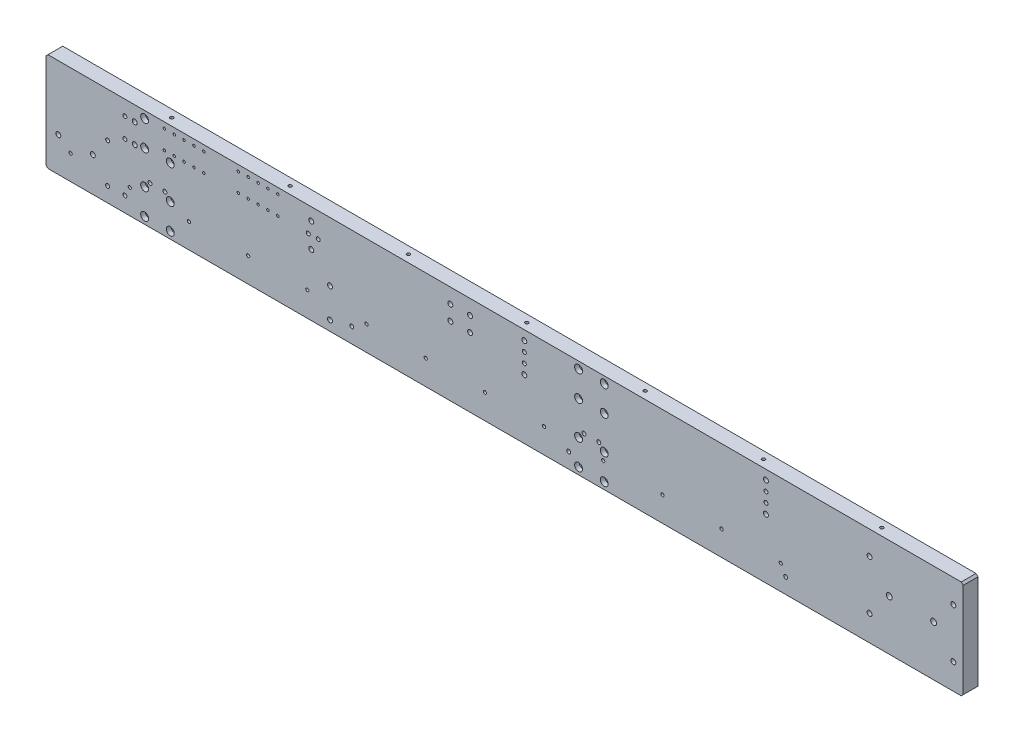
from build123d import *

# Parameters (mm, degrees)
SKETCH2_W                                        = 930
SKETCH2_H                                        = 100
BOSS_EXTRUDE1_DEPTH                              = 15
HOLE_SIZE_PER_HEX_SOCKET_SCREW_TYPE1_D           = 4.5
HOLE_SIZE_PER_HEX_SOCKET_SCREW_TYPE1_CBORE_D     = 8
HOLE_SIZE_PER_HEX_SOCKET_SCREW_TYPE1_CBORE_DEPTH = 4.6
M6_TAPPED_HOLE1_D                                = 5
M6_TAPPED_HOLE1_DEPTH                            = 15
M6_TAPPED_HOLE1_TIP                              = 1.502151548
M6_TAPPED_HOLE2_D                                = 5
M6_TAPPED_HOLE2_DEPTH                            = 15
M6_TAPPED_HOLE2_TIP                              = 1.502151548
LPATTERN2_COUNT                                  = 13
LPATTERN2_PITCH                                  = 60
M3_TAPPED_HOLE1_D                                = 2.5
M3_TAPPED_HOLE1_DEPTH                            = 8.5
M3_TAPPED_HOLE1_TIP                              = 0.751075774
F_4_0_4_DIAMETER_HOLE1_D                         = 4
F_4_0_4_DIAMETER_HOLE1_DEPTH                     = 15
F_4_0_4_DIAMETER_HOLE1_TIP                       = 1.201721238
F_6_0_6_DIAMETER_HOLE1_D                         = 6
F_6_0_6_DIAMETER_HOLE1_DEPTH                     = 15
F_6_0_6_DIAMETER_HOLE1_TIP                       = 1.802581857
M4_TAPPED_HOLE2_D                                = 3.3
M4_TAPPED_HOLE2_DEPTH                            = 11.5
M4_TAPPED_HOLE2_TIP                              = 0.991420021
M4_TAPPED_HOLE3_D                                = 3.3
M4_TAPPED_HOLE3_DEPTH                            = 10.1
M4_TAPPED_HOLE3_TIP                              = 0.991420021
M3_TAPPED_HOLE2_D                                = 2.5
M3_TAPPED_HOLE2_DEPTH                            = 8.5
M3_TAPPED_HOLE2_TIP                              = 0.751075774
CHAMFER1_SIZE                                    = 2


with BuildPart() as part:
    # Sketch2 → Boss-Extrude1 (new body)
    with BuildSketch(Plane.XY):
        with Locations((465, 50)):
            Rectangle(SKETCH2_W, SKETCH2_H)
    extrude(amount=-BOSS_EXTRUDE1_DEPTH)

    # Hole size per hex socket screw type1 (through all)
    with Locations(Plane.XY):
        with Locations((100, 33), (126, 33), (100, 7), (126, 7), (100, 67), (126, 67), (100, 93), (540, 7), (566, 7), (540, 33), (566, 33), (540, 67), (566, 67), (540, 93), (566, 93)):
            CounterBoreHole(HOLE_SIZE_PER_HEX_SOCKET_SCREW_TYPE1_D / 2, HOLE_SIZE_PER_HEX_SOCKET_SCREW_TYPE1_CBORE_D / 2, HOLE_SIZE_PER_HEX_SOCKET_SCREW_TYPE1_CBORE_DEPTH)

    # M6 Tapped Hole1
    with Locations(Plane.XY):
        with Locations((12.5, 35), (47.5, 35), (90, 85), (90, 65), (269, 62.5), (269, 87.5), (835, 76), (920, 76), (920, 26), (835, 26), (410, 85), (410, 70), (430, 85), (430, 70), (485, 90.5), (485, 60.5), (730, 90.5), (730, 60.5), (288, 40), (288, 10)):
            Hole(M6_TAPPED_HOLE1_D / 2, depth=M6_TAPPED_HOLE1_DEPTH)
            with Locations((0, 0, -(M6_TAPPED_HOLE1_DEPTH + M6_TAPPED_HOLE1_TIP / 2))):  # 118° drill point
                Cone(0, M6_TAPPED_HOLE1_D / 2, M6_TAPPED_HOLE1_TIP, mode=Mode.SUBTRACT)

    # M6 Tapped Hole2
    with Locations(Plane(origin=(0, 0, 0), x_dir=(-1, 0, 0), z_dir=(0, -1, 0))):
        with Locations((-340, 7.5), (-385, 7.5)):
            Hole(M6_TAPPED_HOLE2_D / 2, depth=M6_TAPPED_HOLE2_DEPTH)
            with Locations((0, 0, -(M6_TAPPED_HOLE2_DEPTH + M6_TAPPED_HOLE2_TIP / 2))):  # 118° drill point
                Cone(0, M6_TAPPED_HOLE2_D / 2, M6_TAPPED_HOLE2_TIP, mode=Mode.SUBTRACT)

    # Sketch9 → M4 Tapped Hole1 (revolve, cut)
    with BuildSketch(Plane(origin=(25, 25, 0), x_dir=(0, -1, 0), z_dir=(1, 0, 0))):
        Polygon((0, 0), (0, 11.091420021), (1.65, 10.1), (1.65, 0), align=None)
    m4_tapped_hole1 = revolve(axis=Axis((25, 25, 6.35), (0, 0, -1)), mode=Mode.SUBTRACT)

    # LPattern2: M4 Tapped Hole1 ×13
    with Locations(*[(i * LPATTERN2_PITCH, 0, 0) for i in range(1, LPATTERN2_COUNT)]):
        add(m4_tapped_hole1, mode=Mode.SUBTRACT)

    # M3 Tapped Hole1
    with Locations(Plane.XY):
        with Locations((120, 94), (120, 75), (130, 94), (130, 75), (140, 94), (140, 75), (235, 94), (235, 75), (225, 94), (225, 75), (215, 94), (215, 75), (150, 94), (160, 94), (205, 94), (195, 94), (150, 75), (160, 75), (195, 75), (205, 75)):
            Hole(M3_TAPPED_HOLE1_D / 2, depth=M3_TAPPED_HOLE1_DEPTH)
            with Locations((0, 0, -(M3_TAPPED_HOLE1_DEPTH + M3_TAPPED_HOLE1_TIP / 2))):  # 118° drill point
                Cone(0, M3_TAPPED_HOLE1_D / 2, M3_TAPPED_HOLE1_TIP, mode=Mode.SUBTRACT)

    # Ø4.0 (4) Diameter Hole1
    with Locations(Plane.XY):
        with Locations((62.5, 55), (62.5, 15), (80, 65), (80, 85), (80, 15.5), (310, 15.5), (485, 70.5), (485, 80.5), (730, 80.5), (730, 70.5), (266, 75), (276, 75), (105.5, 39), (120.5, 39), (545.5, 39), (560.5, 39), (750, 15.5), (530, 15.5)):
            Hole(F_4_0_4_DIAMETER_HOLE1_D / 2, depth=F_4_0_4_DIAMETER_HOLE1_DEPTH)
            with Locations((0, 0, -(F_4_0_4_DIAMETER_HOLE1_DEPTH + F_4_0_4_DIAMETER_HOLE1_TIP / 2))):  # 118° drill point
                Cone(0, F_4_0_4_DIAMETER_HOLE1_D / 2, F_4_0_4_DIAMETER_HOLE1_TIP, mode=Mode.SUBTRACT)

    # Ø6.0 (6) Diameter Hole1
    with Locations(Plane.XY):
        with Locations((855, 51), (900, 51)):
            Hole(F_6_0_6_DIAMETER_HOLE1_D / 2, depth=F_6_0_6_DIAMETER_HOLE1_DEPTH)
            with Locations((0, 0, -(F_6_0_6_DIAMETER_HOLE1_DEPTH + F_6_0_6_DIAMETER_HOLE1_TIP / 2))):  # 118° drill point
                Cone(0, F_6_0_6_DIAMETER_HOLE1_D / 2, F_6_0_6_DIAMETER_HOLE1_TIP, mode=Mode.SUBTRACT)

    # M4 Tapped Hole2
    with Locations(Plane(origin=(0, 100, 0), x_dir=(1, 0, 0), z_dir=(0, 1, 0))):
        with Locations((600, 7.5), (120, 7.5), (240, 7.5), (360, 7.5), (480, 7.5), (720, 7.5), (840, 7.5)):
            Hole(M4_TAPPED_HOLE2_D / 2, depth=M4_TAPPED_HOLE2_DEPTH)
            with Locations((0, 0, -(M4_TAPPED_HOLE2_DEPTH + M4_TAPPED_HOLE2_TIP / 2))):  # 118° drill point
                Cone(0, M4_TAPPED_HOLE2_D / 2, M4_TAPPED_HOLE2_TIP, mode=Mode.SUBTRACT)

    # M4 Tapped Hole3
    with Locations(Plane.ZY):
        with Locations((-7.5, 35), (-7.5, 15)):
            Hole(M4_TAPPED_HOLE3_D / 2, depth=M4_TAPPED_HOLE3_DEPTH)
            with Locations((0, 0, -(M4_TAPPED_HOLE3_DEPTH + M4_TAPPED_HOLE3_TIP / 2))):  # 118° drill point
                Cone(0, M4_TAPPED_HOLE3_D / 2, M4_TAPPED_HOLE3_TIP, mode=Mode.SUBTRACT)

    # M3 Tapped Hole2
    with Locations(Plane(origin=(0, 0, 0), x_dir=(-1, 0, 0), z_dir=(0, -1, 0))):
        with Locations((-110, 7.5), (-150, 7.5)):
            Hole(M3_TAPPED_HOLE2_D / 2, depth=M3_TAPPED_HOLE2_DEPTH)
            with Locations((0, 0, -(M3_TAPPED_HOLE2_DEPTH + M3_TAPPED_HOLE2_TIP / 2))):  # 118° drill point
                Cone(0, M3_TAPPED_HOLE2_D / 2, M3_TAPPED_HOLE2_TIP, mode=Mode.SUBTRACT)

    # Chamfer1
    chamfer1_edges = [part.edges().sort_by_distance(p)[0] for p in [
        (930, 0, -7.5),
        (0, 0, -7.5),
        (0, 100, -7.5),
        (930, 100, -7.5),
    ]]
    chamfer(chamfer1_edges, length=CHAMFER1_SIZE)


solid = part.part
